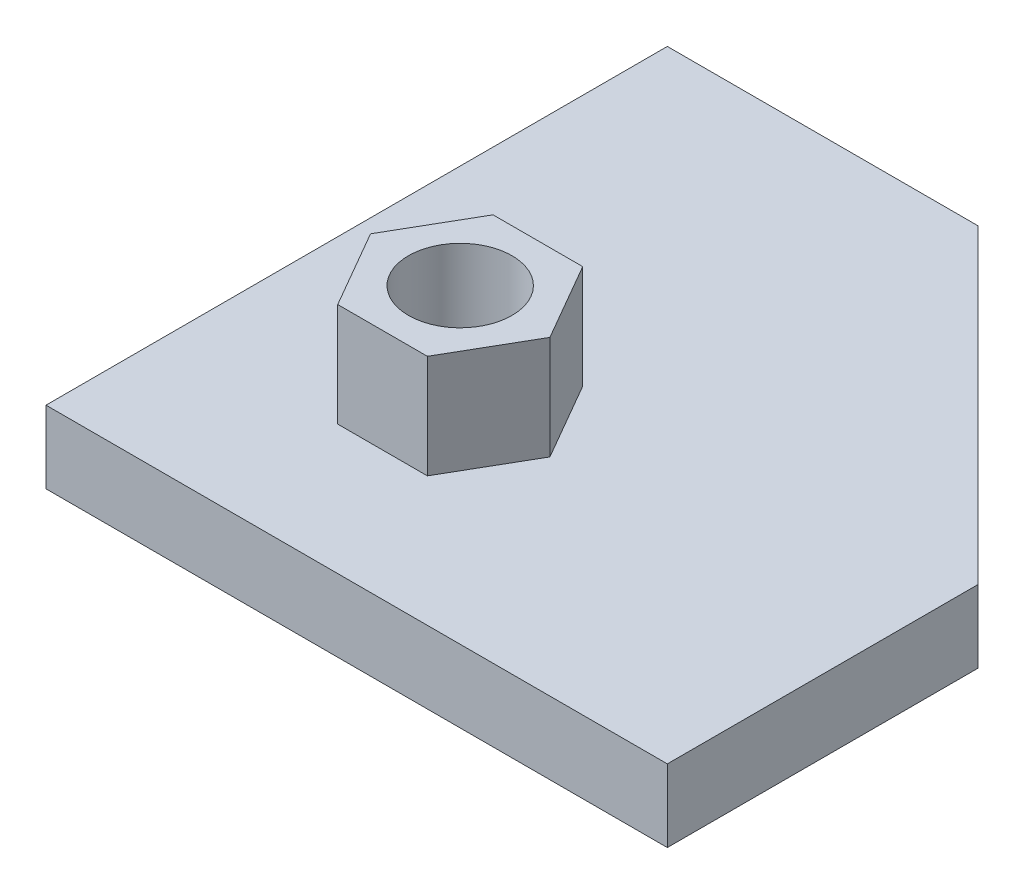
from build123d import *

# Parameters (mm, degrees)
BOSS_EXTRUDE1_DEPTH = 14
SKETCH3_R           = 11.5
CUT_EXTRUDE1_DEPTH  = 14
SKETCH4_R           = 10
BOSS_EXTRUDE2_DEPTH = 20


with BuildPart() as part:
    # Sketch2 → Boss-Extrude1 (new body)
    with BuildSketch(Plane(origin=(0, 0, 0), x_dir=(1, 0, 0), z_dir=(0, 1, 0))):
        Polygon((0, 0), (0, 120), (60, 120), (120, 60), (120, 0), align=None)
    extrude(amount=BOSS_EXTRUDE1_DEPTH)

    # Sketch3 → Cut-Extrude1 (cut)
    with BuildSketch(Plane(origin=(0, 14, 0), x_dir=(1, 0, 0), z_dir=(0, 1, 0))):
        with Locations(Location((40, 40, 0), (0, 0, 270))):
            Circle(SKETCH3_R)
    extrude(amount=-CUT_EXTRUDE1_DEPTH, mode=Mode.SUBTRACT)

    # Sketch4 → Boss-Extrude2 (add)
    with BuildSketch(Plane(origin=(0, 14, 0), x_dir=(1, 0, 0), z_dir=(0, 1, 0))):
        Polygon((57.320508076, 40), (48.660254038, 55), (31.339745962, 55), (22.679491924, 40), (31.339745962, 25), (48.660254038, 25), align=None)
        with Locations(Location((40, 40, 0), (0, 0, 270))):
            Circle(SKETCH4_R, mode=Mode.SUBTRACT)
    extrude(amount=BOSS_EXTRUDE2_DEPTH)


solid = part.part
